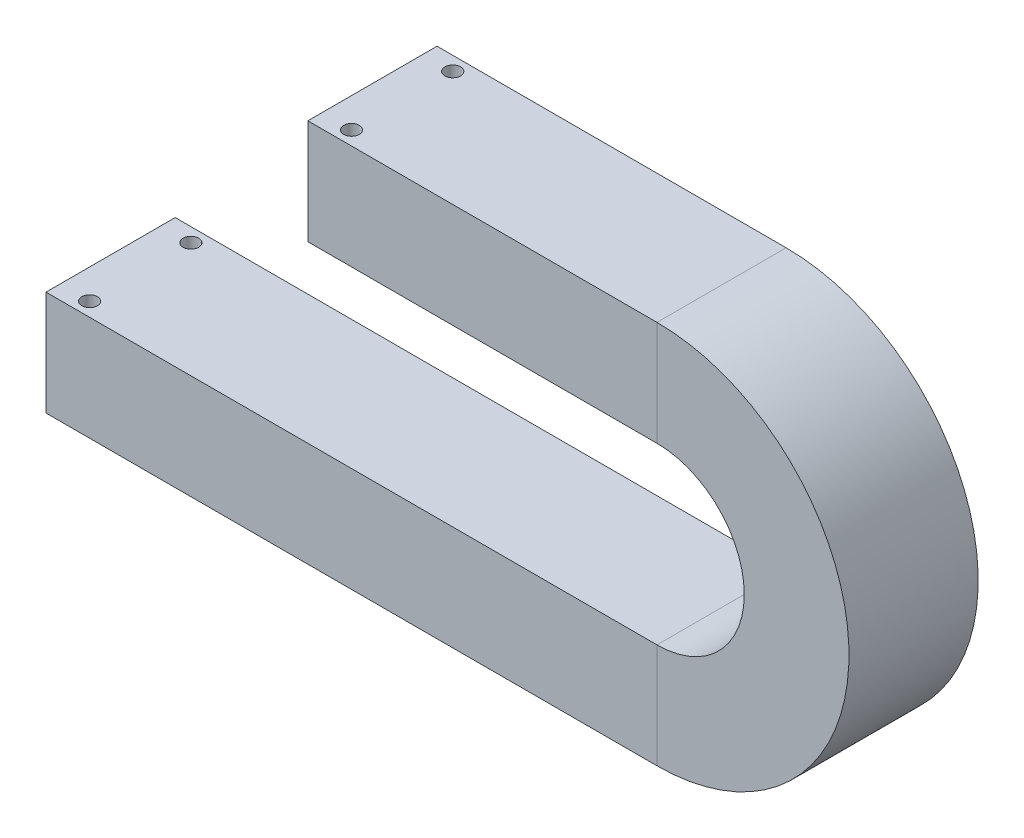
from build123d import *

# Parameters (mm, degrees)
SKETCH1_W                = 37
SKETCH1_H                = 30
SKETCH1_W_2              = 20
SKETCH1_H_2              = 20
M4_CLEARANCE_HOLE1_D     = 4.5
M4_CLEARANCE_HOLE2_D     = 4.5
M4_CLEARANCE_HOLE2_DEPTH = 50
M4_CLEARANCE_HOLE2_TIP   = 1.351936393


with BuildPart() as part:
    # Sweep1: sweep along a path in Sketch2
    with BuildLine(Plane.XY) as sweep1_path:
        Line((0, 0), (175, 0))
        ThreePointArc((175, 0), (215, 40), (175, 80))
        Line((175, 80), (75, 80))
    # Sketch1 → Sweep1 (sweep)
    with BuildSketch(Plane(origin=(0, 0, 0), x_dir=(0, 0, -1), z_dir=(1, 0, 0))):
        Rectangle(SKETCH1_W, SKETCH1_H)
        Rectangle(SKETCH1_W_2, SKETCH1_H_2, mode=Mode.SUBTRACT)
    sweep(path=sweep1_path.line)

    # M4 Clearance Hole1 (through all)
    with Locations(Plane(origin=(0, 15, 0), x_dir=(1, 0, 0), z_dir=(0, 1, 0))):
        with Locations((8.5, 14.5), (8.5, -14.5)):
            Hole(M4_CLEARANCE_HOLE1_D / 2)

    # M4 Clearance Hole2
    with Locations(Plane(origin=(0, 95, 0), x_dir=(1, 0, 0), z_dir=(0, 1, 0))):
        with Locations((83.5, -14.5), (83.5, 14.5)):
            Hole(M4_CLEARANCE_HOLE2_D / 2, depth=M4_CLEARANCE_HOLE2_DEPTH)
            with Locations((0, 0, -(M4_CLEARANCE_HOLE2_DEPTH + M4_CLEARANCE_HOLE2_TIP / 2))):  # 118° drill point
                Cone(0, M4_CLEARANCE_HOLE2_D / 2, M4_CLEARANCE_HOLE2_TIP, mode=Mode.SUBTRACT)


solid = part.part
